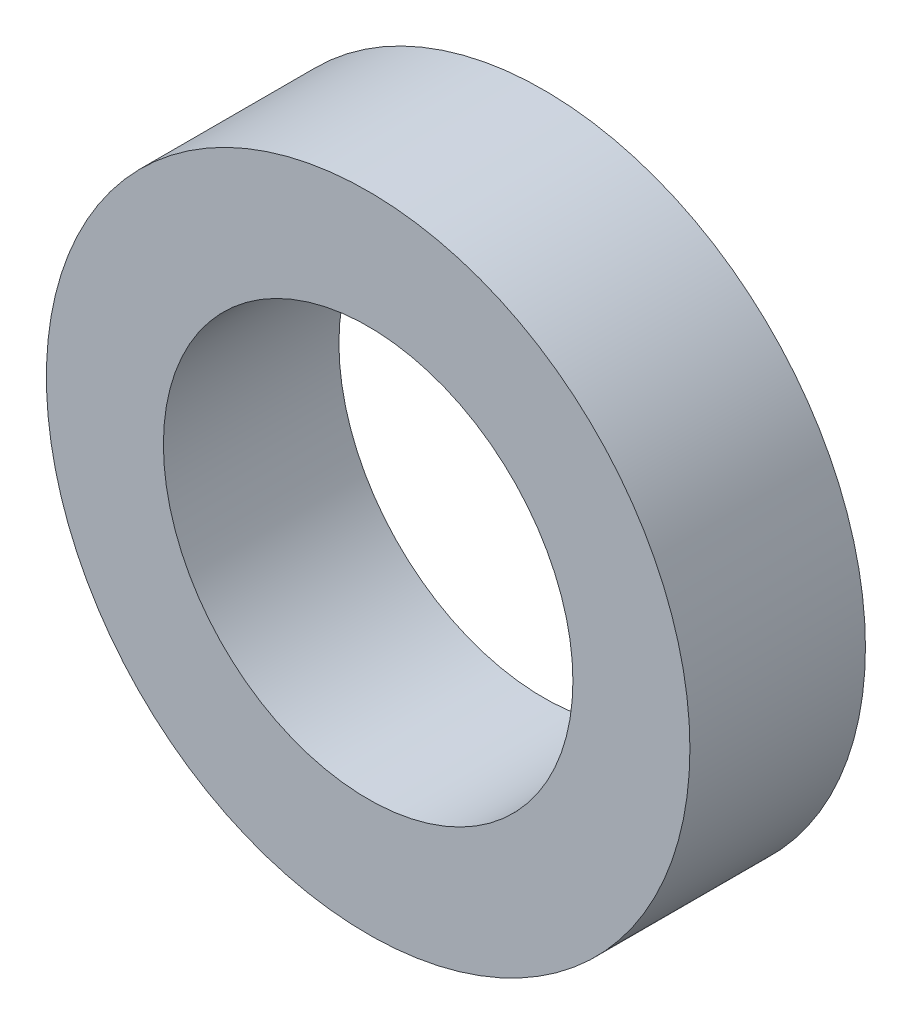
SolidWorks part; units mm, degrees
ref_plane "Front Plane" through (0, 0, 0) normal (0, 0, 1) x (1, 0, 0)
ref_plane "Top Plane" through (0, 0, 0) normal (0, 1, 0) x (1, 0, 0)
ref_plane "Right Plane" through (0, 0, 0) normal (1, 0, 0) x (0, 0, -1)
other "Configuration Table"
sketch "Sketch1" plane through (0, 0, 0) normal (1, 0, 0) x (0, 0, -1)
  line L4 (-4.5484, 0) -> (15.0294, 0) construction
  line L5 (0, 7) -> (0, 11)
  line L6 (0, 11) -> (6, 11)
  line L7 (6, 11) -> (6, 7)
  line L8 (6, 7) -> (0, 7)
  dimension "D1" = 7
  dimension "D2" = 6
  dimension "D3" = 11
revolve "Revolve1" add sketch "Sketch1" angle 360 about L4
